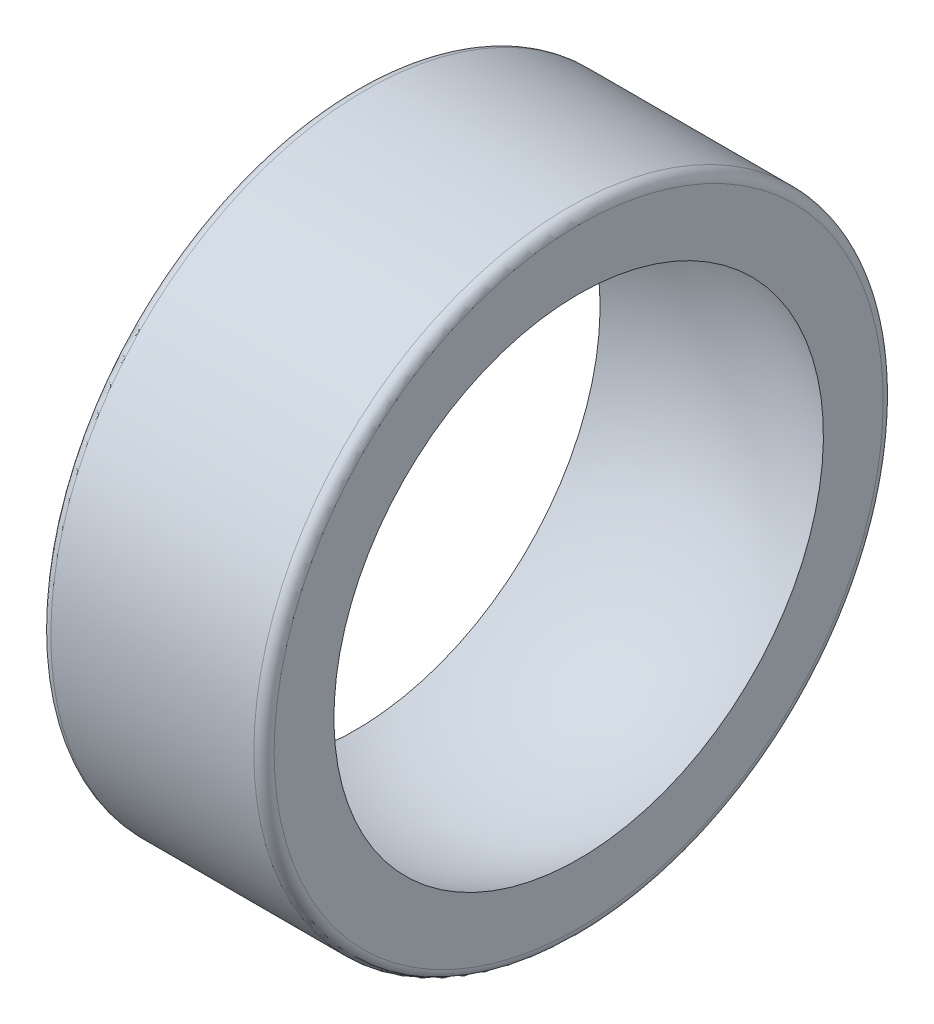
SolidWorks part; units mm, degrees
material "普通碳钢"
ref_plane "前视" through (0, 0, 0) normal (0, 0, 1) x (1, 0, 0)
ref_plane "上视" through (0, 0, 0) normal (0, 1, 0) x (1, 0, 0)
ref_plane "右视" through (0, 0, 0) normal (1, 0, 0) x (0, 0, -1)
sketch "草图2" plane through (0, 0, 0) normal (0, 0, 1) x (1, 0, 0)
  line L0 (-53.0125, 0) -> (57.5349, 0) construction
  line L1 (0, 35.551) -> (0, -36.3048) construction
  line L2 (-11, 31) -> (-11, 24.1091)
  line L3 (11, 31) -> (11, 24.1091)
  line L4 (-11, 31) -> (11, 31)
  arc A1 (11, 24.1091) -> (-11, 24.1091) centre (0, 0) ccw
  dimension "D1" = 26.5
  dimension "D2" = 22
  dimension "D3" = 31
revolve "旋转1" add sketch "草图2" angle 360 about L0
fillet "圆角1" radius 1 2 edges at (-11, 0, 31) (11, 0, 31)
